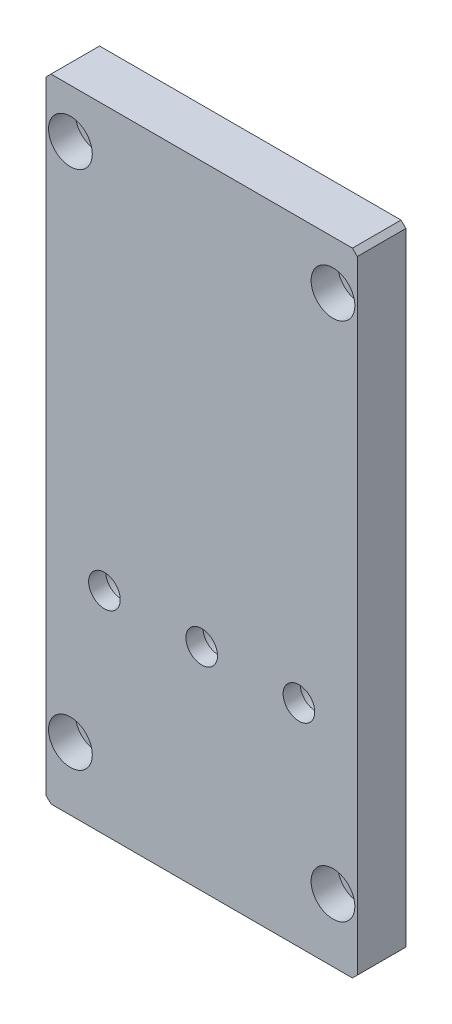
SolidWorks part; units mm, degrees
material "6061-T6 (SS)"
ref_plane "前视基准面" through (0, 0, 0) normal (0, 0, 1) x (1, 0, 0)
ref_plane "上视基准面" through (0, 0, 0) normal (0, 1, 0) x (1, 0, 0)
ref_plane "右视基准面" through (0, 0, 0) normal (1, 0, 0) x (0, 0, -1)
sketch "草图1" plane through (0, 0, 0) normal (0, 0, 1) x (1, 0, 0)
  line L0 (-22, 0) -> (42, 0)
  line L1 (42, 0) -> (42, -130)
  line L3 (42, -130) -> (-22, -130)
  line L5 (-22, -130) -> (-22, 0)
  dimension "D1" = 130
  dimension "D2" = 64
extrude "凸台-拉伸1" add sketch "草图1" along normal blind 10
hole_wizard "打孔尺寸根据内六角圆柱头螺钉的类型0" positions "草图3" profile "草图2" counterbore size "M5" standard "Gb" end condition through all
sketch "草图3" plane through (0, 0, 10) normal (0, 0, 1) x (1, 0, 0)
  point P0 (-17, -10)
  point P3 (37, -10)
  point P6 (-17, -117)
  point P9 (37, -117)
sketch "草图2" plane through (-17, -10, 10) normal (1, 0, 0) x (0, -1, 0)
  line L0 (0, 0) -> (0, 10)
  line L1 (0, 10) -> (2.75, 10)
  line L3 (2.75, 10) -> (2.75, 5.5)
  line L4 (2.75, 5.5) -> (4.5, 5.5)
  line L5 (4.5, 5.5) -> (4.5, 0)
  line L7 (4.5, 0) -> (0, 0)
  line L11 (0, -6.35) -> (0, 107.95) construction
  dimension "通孔孔直径" = 5.5
  dimension "通孔孔深度" = 10
  dimension "柱形沉头孔直径" = 9
  dimension "柱形沉头孔深度" = 5.5
hole_wizard "打孔尺寸根据六角头螺栓 C 级的类型1" positions "草图5" profile "草图4" counterbore size "M6" standard "Gb" end condition through all
sketch "草图5" plane through (0, 0, 0) normal (0, 0, -1) x (-1, 0, 0)
  line L0 (22, -130) -> (-42, -130) construction
  point P0 (10, -86.5)
  point P3 (-10, -86.5)
  point P6 (-30, -86.5)
  dimension "D1" = 43.5
sketch "草图4" plane through (-10, -86.5, 0) normal (1, 0, 0) x (0, 1, 0)
  line L0 (0, 0) -> (0, 10)
  line L1 (0, 10) -> (3.25, 10)
  line L3 (3.25, 10) -> (3.25, 6.5)
  line L4 (3.25, 6.5) -> (6, 6.5)
  line L5 (6, 6.5) -> (6, 0)
  line L7 (6, 0) -> (0, 0)
  line L11 (0, -6.35) -> (0, 107.95) construction
  dimension "通孔孔直径" = 6.5
  dimension "通孔孔深度" = 10
  dimension "柱形沉头孔直径" = 12
  dimension "柱形沉头孔深度" = 6.5
chamfer "倒角1" distance 1 angle 45 4 edges at (42, -130, 5) (-22, -130, 5) (-22, 0, 5) (42, 0, 5)
